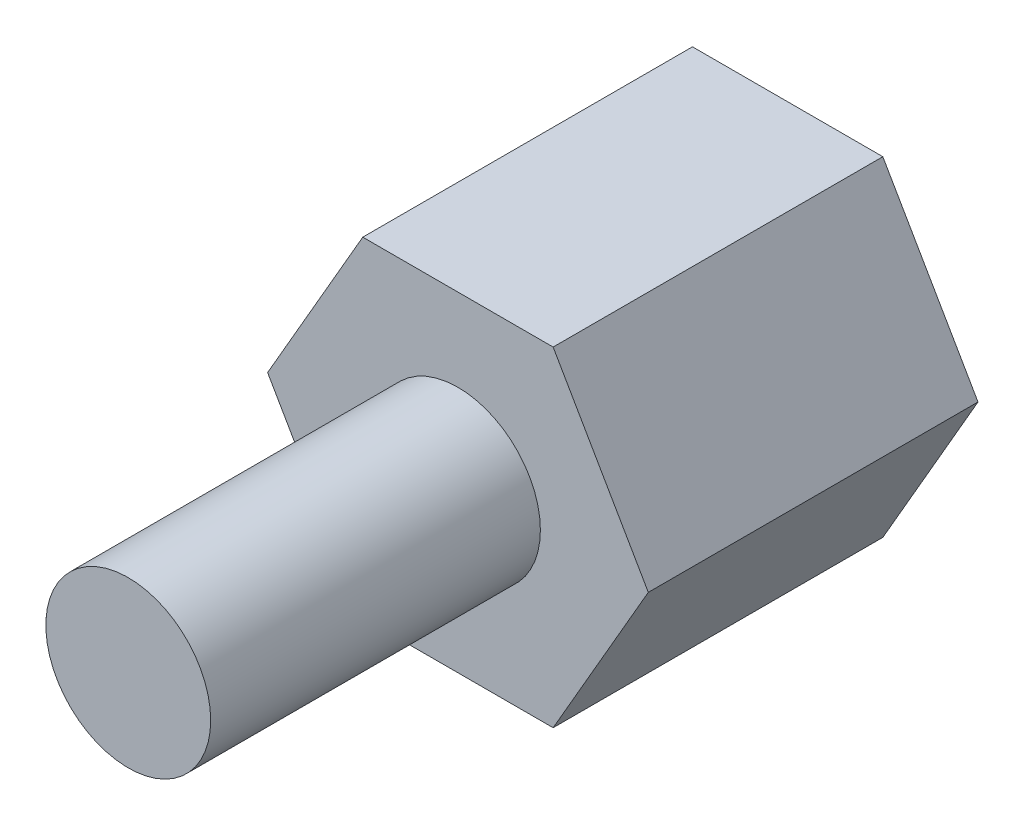
SolidWorks part; units mm, degrees
ref_plane "前视基准面" through (0, 0, 0) normal (0, 0, 1) x (1, 0, 0)
ref_plane "上视基准面" through (0, 0, 0) normal (0, 1, 0) x (1, 0, 0)
ref_plane "右视基准面" through (0, 0, 0) normal (1, 0, 0) x (0, 0, -1)
sketch "草图1" plane through (0, 0, 0) normal (0, 0, 1) x (1, 0, 0)
  line L1 (3.4641, 0) -> (1.7321, 3)
  line L2 (1.7321, 3) -> (-1.7321, 3)
  line L3 (-1.7321, 3) -> (-3.4641, 0)
  line L4 (-3.4641, 0) -> (-1.7321, -3)
  line L5 (-1.7321, -3) -> (1.7321, -3)
  line L6 (1.7321, -3) -> (3.4641, 0)
  circle A0 centre (0, 0) radius 3 construction
  dimension "D1" = 6
extrude "凸台-拉伸1" add sketch "草图1" along normal blind 6
sketch "草图2" plane through (0, 0, 6) normal (0, 0, 1) x (1, 0, 0)
  circle A0 centre (0, 0) radius 1.5
  dimension "D1" = 3
extrude "凸台-拉伸2" add sketch "草图2" along normal blind 6
sketch "草图3" plane through (0, 0, 0) normal (0, 0, -1) x (-1, 0, 0)
  circle A0 centre (0, 0) radius 1.5
  dimension "D1" = 3
extrude "切除-拉伸1" cut sketch "草图3" against normal blind 3
